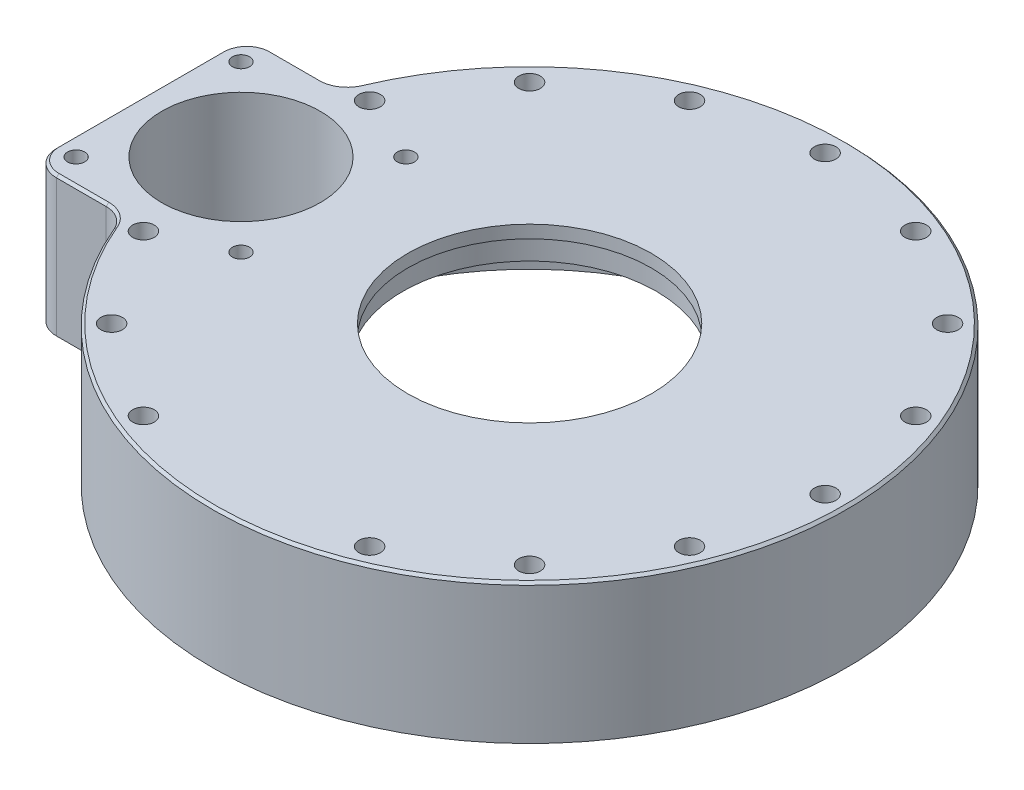
SolidWorks part; units mm, degrees
material "Q235A"
ref_plane "前视基准面" through (0, 0, 0) normal (0, 0, 1) x (1, 0, 0)
ref_plane "上视基准面" through (0, 0, 0) normal (0, 1, 0) x (1, 0, 0)
ref_plane "右视基准面" through (0, 0, 0) normal (1, 0, 0) x (0, 0, -1)
sketch "草图2" plane through (0, 0, 0) normal (0, 0, 1) x (1, 0, 0)
  line L0 (0, 0) -> (0, 174.2349) construction
  line L2 (104, 0) -> (104, 41)
  line L3 (104, 41) -> (50, 41)
  line L4 (50, 41) -> (50, 50)
  line L5 (50, 50) -> (48, 50)
  line L6 (48, 50) -> (48, 55)
  line L7 (48, 55) -> (125, 55)
  line L8 (125, 55) -> (125, 0)
  line L9 (125, 0) -> (104, 0)
  dimension "D1" = 250
  dimension "D2" = 208
  dimension "D3" = 2
  dimension "D4" = 41
  dimension "D5" = 100
  dimension "D7" = 50
  dimension "D8" = 5
revolve "旋转1" add sketch "草图2" angle 360 about L0
sketch "草图3" plane through (0, 55, 0) normal (0, 1, 0) x (1, 0, 0)
  line L1 (-104, -42.5) -> (-154, -42.5)
  line L2 (-104, -42.5) -> (-104, 42.5)
  line L3 (-104, 42.5) -> (-154, 42.5)
  line L4 (-154, -42.5) -> (-154, 42.5)
  line L5 (-104, -42.5) -> (-154, 42.5) construction
  line L6 (-104, 42.5) -> (-154, -42.5) construction
  circle A2 centre (0, 0) radius 104 construction
  point P0 (-129, 0)
  dimension "D1" = 50
  dimension "D2" = 85
extrude "凸台-拉伸1" add sketch "草图3" against normal through all
sketch "草图5" plane through (0, 55, 0) normal (0, 1, 0) x (1, 0, 0)
  circle A0 centre (-113.75, 0) radius 31.25
  dimension "D1" = 113.75
  dimension "D2" = 62.5
extrude "切除-拉伸1" cut sketch "草图5" against normal offset from surface (45 mm away) 10 up to face at (0, 0, -104)
hole_wizard "M8 螺纹孔1" positions "草图6" profile "草图7" tap size "M8" standard "ISO"
sketch "草图6" plane through (0, 55, 0) normal (0, 1, 0) x (1, 0, 0)
  line L1 (-146.25, -32.5) -> (-81.25, -32.5)
  line L2 (-146.25, -32.5) -> (-146.25, 32.5)
  line L3 (-146.25, 32.5) -> (-81.25, 32.5)
  line L4 (-81.25, -32.5) -> (-81.25, 32.5)
  line L5 (-146.25, -32.5) -> (-81.25, 32.5) construction
  line L6 (-146.25, 32.5) -> (-81.25, -32.5) construction
  point P0 (-146.25, 32.5)
  point P3 (-113.75, 0)
  point P4 (-81.25, 32.5)
  point P7 (-146.25, -32.5)
  point P9 (-81.25, -32.5)
  dimension "D1" = 65
sketch "草图7" plane through (-146.25, 55, -32.5) normal (1, 0, 0) x (0, 0, 1)
  line L0 (0, 0) -> (0, 21.7929)
  line L1 (0, 21.7929) -> (3.4, 19.75)
  line L2 (3.4, 19.75) -> (3.4, 0)
  line L5 (3.4, 0) -> (0, 0)
  line L10 (0, 21.7929) -> (-3.4, 19.75) construction
  line L11 (0, -6.35) -> (0, 107.95) construction
  dimension "螺纹孔钻头直径" = 6.8
  dimension "螺纹孔钻头深度" = 19.75
  dimension "导头角度" = 118
cosmetic thread "孔螺蚊线1" parameters "D1"=16, "D2"=8
cosmetic thread "孔螺蚊线2" parameters "D1"=16, "D2"=8
cosmetic thread "孔螺蚊线3" parameters "D1"=16, "D2"=8
cosmetic thread "孔螺蚊线4" parameters "D1"=16, "D2"=8
fillet "圆角1" radius 10 4 edges at (-154, 27.5, 42.5) (-154, 27.5, -42.5) (-117.5532, 27.5, -42.5) (-117.5532, 27.5, 42.5)
hole_wizard "M10 螺纹孔1" positions "草图8" profile "草图9" tap size "M10" standard "ISO" end condition through all
sketch "草图8" plane through (0, 0, 0) normal (0, -1, 0) x (-1, 0, 0)
  line L0 (0, 0) -> (-107.632, -44.5826) construction
  line L1 (0, 0) -> (154, 0) construction
  line L2 (154, 32.5) -> (154, -32.5) construction
  point P0 (-107.632, -44.5826)
  point P6 (-107.632, 44.5826)
  point P7 (-44.5826, 107.632)
  point P8 (44.5826, 107.632)
  point P9 (107.632, 44.5826)
  point P10 (107.632, -44.5826)
  point P11 (44.5826, -107.632)
  point P12 (-44.5826, -107.632)
  point P27 (0, 116.5)
  point P30 (-82.3779, 82.3779)
  point P33 (82.3779, 82.3779)
  point P36 (-82.3779, -82.3779)
  point P39 (82.3779, -82.3779)
  point P42 (-116.5, 0)
  dimension "D2" = 116.5
  dimension "D3" = 82.3779
  dimension "D4" = 82.3779
  dimension "D5" = 116.5
  dimension "D6" = 82.3779
  dimension "D7" = 116.5
  dimension "D8" = 82.3779
  dimension "D1" = 8
cosmetic thread "孔螺蚊线5" parameters "D2"=10
cosmetic thread "孔螺蚊线6" parameters "D2"=10
cosmetic thread "孔螺蚊线7" parameters "D2"=10
cosmetic thread "孔螺蚊线8" parameters "D2"=10
cosmetic thread "孔螺蚊线9" parameters "D2"=10
cosmetic thread "孔螺蚊线10" parameters "D2"=10
cosmetic thread "孔螺蚊线11" parameters "D2"=10
cosmetic thread "孔螺蚊线12" parameters "D2"=10
cosmetic thread "孔螺蚊线13" parameters "D2"=10
cosmetic thread "孔螺蚊线14" parameters "D2"=10
cosmetic thread "孔螺蚊线15" parameters "D2"=10
cosmetic thread "孔螺蚊线16" parameters "D2"=10
cosmetic thread "孔螺蚊线17" parameters "D2"=10
cosmetic thread "孔螺蚊线18" parameters "D2"=10
sketch "草图9" plane through (107.632, 0, 44.5826) normal (1, 0, 0) x (0, 0, -1)
  line L0 (0, 0) -> (0, 55)
  line L1 (0, 55) -> (4.25, 55)
  line L2 (4.25, 55) -> (4.25, 0)
  line L5 (4.25, 0) -> (0, 0)
  line L11 (0, -6.35) -> (0, 107.95) construction
  dimension "通孔螺纹孔钻头直径" = 8.5
  dimension "通孔螺纹孔钻头深度" = 55
chamfer "倒角1" distance 1 angle 45 8 edges at (-154, 55, 0) (-151.0711, 55, -39.5711) (-151.0711, 55, 39.5711) (-134.1867, 55, -42.5) (-134.1867, 55, 42.5) (-118.8457, 55, -44.1667) (-118.8457, 55, 44.1667) (125, 55, 0)
